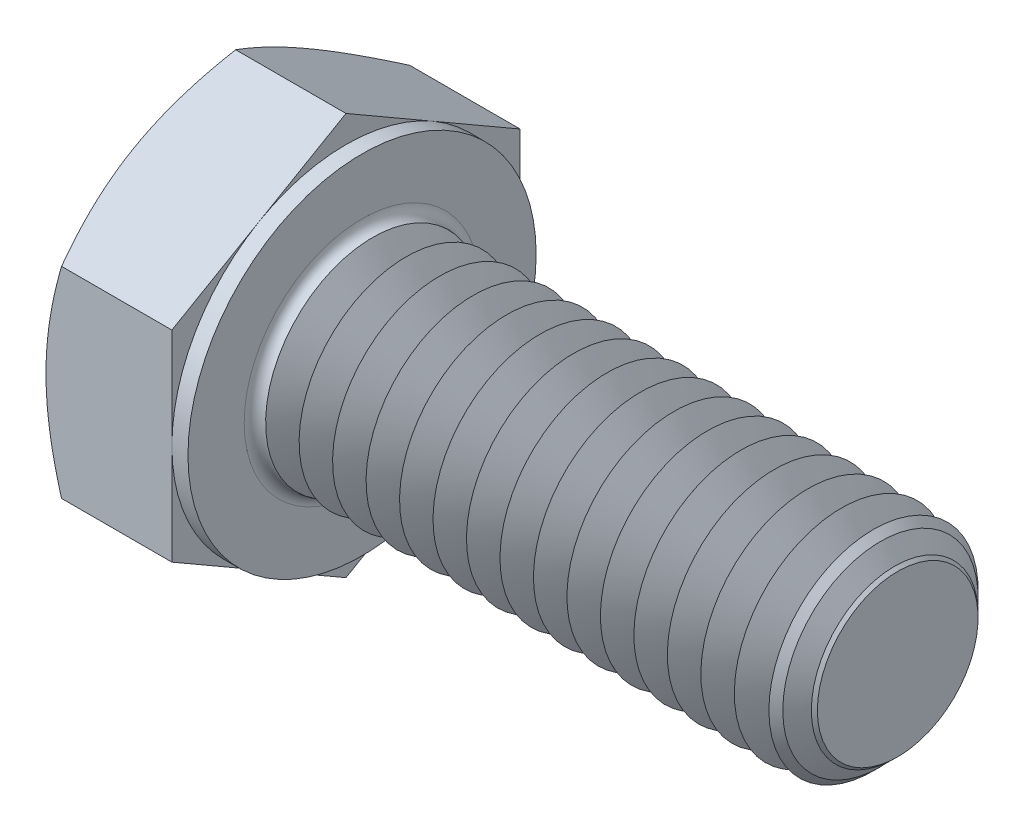
SolidWorks part; units mm, degrees
extrude "基体-拉伸" add sketch "草图1" along normal blind 5.3
sketch "草图1" plane through (0, 0, 0) normal (1, 0, 0) x (0, 0, -1)
  line L0 (6.5, 3.7528) -> (6.5, -3.7528)
  line L1 (-6.5, 3.7528) -> (-6.5, -3.7528)
  line L2 (6.5, -3.7528) -> (0, -7.5056)
  line L3 (0, -7.5056) -> (-6.5, -3.7528)
  line L4 (6.5, 3.7528) -> (0, 7.5056)
  line L5 (0, 7.5056) -> (-6.5, 3.7528)
revolve "切除-旋转1" cut sketch "草图3" angle 360 about L6
sketch "草图3" plane through (0, 0, 0) normal (0, 0, 1) x (1, 0, 0)
  line L0 (0, 6.5) -> (3.4673, 12.5056)
  line L1 (0, 7.5056) -> (0, 3.7528) construction
  line L2 (3.4673, 12.5056) -> (3.4673, 17.5056)
  line L3 (3.4673, 17.5056) -> (-10, 17.5056)
  line L4 (-10, 17.5056) -> (-10, 6.5)
  line L5 (-10, 6.5) -> (0, 6.5)
  line L6 (0, 0) -> (99.06, 0) construction
  line L7 (5.3, 7.5056) -> (0, 7.5056) construction
revolve "凸台-旋转1" add sketch "草图2" angle 360 about L7
sketch "草图2" plane through (0, 0, 0) normal (0, 0, 1) x (1, 0, 0)
  line L0 (0, 3.7528) -> (0, -3.7528) construction
  line L1 (0, 0) -> (25.3, 0)
  line L2 (0, 0) -> (0, 4)
  line L3 (0, 4) -> (25.3, 4)
  line L4 (25.3, 0) -> (25.3, 2.9175)
  line L5 (5.3, 7.5056) -> (5.3, 3.7528) construction
  line L7 (0, 0) -> (96.52, 0) construction
  line L8 (25.3, -2.9175) -> (90.335, -4) construction
  line L9 (0, -4) -> (90.335, -4) construction
  line L10 (6.55, 15.24) -> (6.55, -1.27) construction
  line L11 (5.3, 15.24) -> (5.3, -1.27) construction
  line L12 (5.3, 3.7528) -> (5.3, -3.7528) construction
  line L14 (25.3, 4) -> (25.3, 2.9175)
  dimension "l" = 20
  dimension "m" = 8
  dimension "Minor_dia" = 5.835
  dimension "p" = 1.25
  dimension "h" = 20
cosmetic thread "螺旋线1" parameters "Thread_length"=18.75, "Thread_minor"=5.835
material "5.6级"
ref_plane "前视" through (0, 0, 0) normal (0, 0, 1) x (1, 0, 0)
ref_plane "上视" through (0, 0, 0) normal (0, 1, 0) x (1, 0, 0)
ref_plane "右视" through (0, 0, 0) normal (1, 0, 0) x (0, 0, -1)
sketch "草图5" plane through (0, 0, 0) normal (0, 0, 1) x (1, 0, 0)
  line L0 (5.3, 6.5) -> (1.8327, 12.5056)
  line L1 (5.3, 7.5056) -> (5.3, 3.7528) construction
  line L2 (1.8327, 12.5056) -> (1.8327, 17.5056)
  line L3 (1.8327, 17.5056) -> (11.8327, 17.5056)
  line L4 (11.8327, 17.5056) -> (11.8327, 6.5)
  line L5 (11.8327, 6.5) -> (5.3, 6.5)
  line L7 (5.3, 7.5056) -> (0.5806, 7.5056) construction
  line L8 (0, 0) -> (99.06, 0) construction
  line L9 (0, 0) -> (99.06, 0) construction
revolve "切除-旋转2" cut sketch "草图5" angle 360 about L8
sketch "草图4" plane through (0, 0, 0) normal (0, 0, 1) x (1, 0, 0)
  line L1 (5.3, 7.5056) -> (5.3, 3.7528) construction
  line L2 (5.3, 6.5) -> (4.7, 6.5)
  line L3 (5.3, 6.5) -> (5.3, 17.5056)
  line L4 (5.3, 17.5056) -> (4.7, 17.5056)
  line L5 (0, 0) -> (95.25, 0) construction
  line L6 (0, 0) -> (96.52, 0) construction
  line L7 (4.7, 6.5) -> (4.7, 17.5056)
  line L8 (4.7194, 7.5056) -> (0.5806, 7.5056) construction
revolve "切除-旋转3" cut sketch "草图4" angle 360 about L5
chamfer "倒角" distance 1 angle 45 1 edges at (25.3, 0, 4)
fillet "圆角" radius 0.4 1 edges at (5.3, 0, -4)
sketch "草图6" plane through (0, 0, 0) normal (0, 0, 1) x (1, 0, 0)
  line L0 (6.325, -2.9175) -> (5.7, -4)
  line L1 (6.325, -2.9175) -> (6.95, -4)
  line L2 (6.95, -4) -> (6.95, -5)
  line L3 (-3.175, 0) -> (5.1513, 0) construction
  line L5 (6.95, -5) -> (5.7, -5)
  line L6 (5.7, -5) -> (5.7, -4)
  arc A0 (5.7, -4) -> (5.3, -4.4) centre (5.7, -4.4) ccw construction
revolve "切除-旋转4" cut sketch "草图6" angle 360 about L3
pattern_linear "阵列(线性)1" count 16 spacing 1.25 along (1, 0, 0) of "切除-旋转4"
equation "\"D3@草图1\" = \"s@草图1\" / 2"
equation "\"D4@草图1\" = \"D3@草图1\""
equation "\"D5@草图1\" = \"D4@草图1\""
equation "\"D1@草图3\" = \"s@草图1\" / 2"
equation "\"D1@草图5\" = \"s@草图1\" / 2"
equation "\"Head_ch_ang@草图5\" = \"Head_ch_ang@草图3\""
equation "\"D1@草图4\" = \"s@草图1\""
equation "\"Diameter@草图6\" = \"m@草图2\""
equation "\"Overcut@草图6\" = \"m@草图2\" * 1.25"
equation "\"Minor_dia@草图2\" = \"m@草图2\"-\"p@草图2\" * 1.732"
equation "\"Thread_minor@螺旋线1\" = \"Minor_dia@草图2\""
equation "\"Thread_minor@草图6\" = \"Minor_dia@草图2\""
equation "\"D1@倒角\" = \"p@草图2\"*0.8"
equation "\"Thread_length@螺旋线1\" = \"l@草图2\" - \"p@草图2\""
equation "\"Num_threads@阵列(线性)1\" = \"l@草图2\" / \"p@草图2\""
